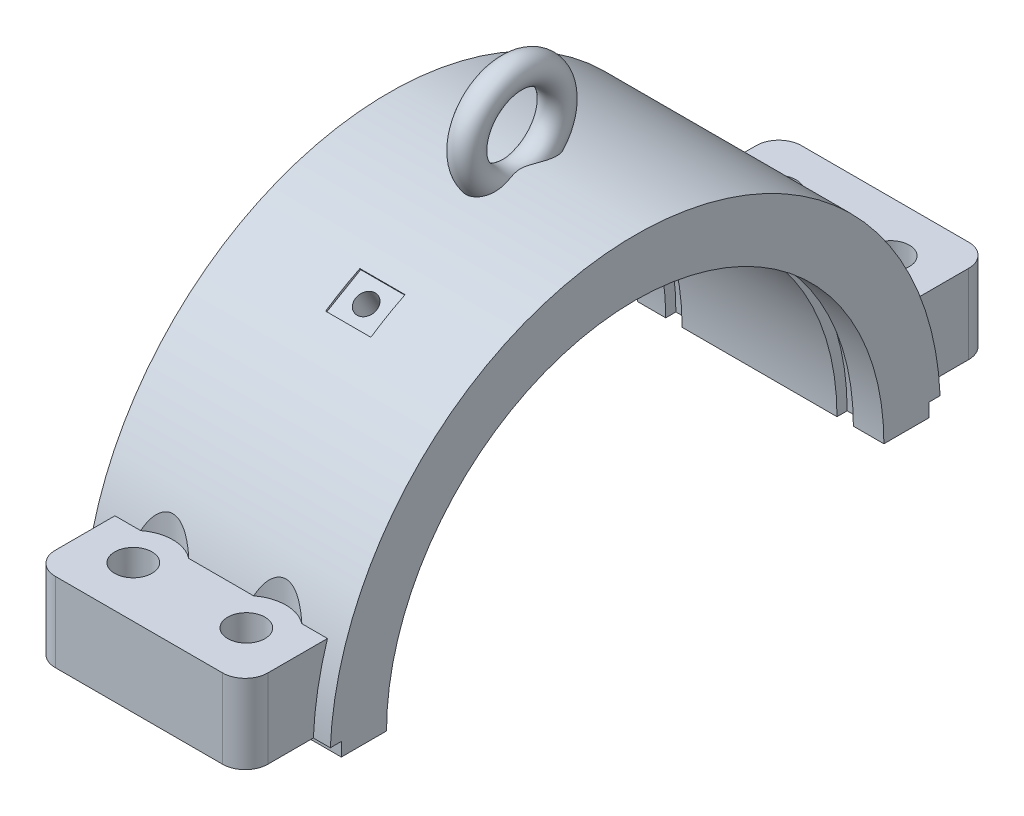
SolidWorks part; units mm, degrees
material "ZG270-500"
ref_plane "Front Plane" through (0, 0, 0) normal (0, 0, 1) x (1, 0, 0)
ref_plane "Top Plane" through (0, 0, 0) normal (0, 1, 0) x (1, 0, 0)
ref_plane "Right Plane" through (0, 0, 0) normal (1, 0, 0) x (0, 0, -1)
sketch "Sketch1" plane through (0, 0, 0) normal (1, 0, 0) x (0, 0, -1)
  line L0 (-323.4956, 0) -> (323.4956, 0) construction
  line L1 (0, 0) -> (0, 289.8169) construction
  line L2 (-270, 0) -> (-220, 0)
  line L3 (220, 0) -> (270, 0)
  arc A0 (220, 0) -> (-220, 0) centre (0, 0) ccw
  arc A1 (270, 0) -> (-270, 0) centre (0, 0) ccw
  point P3 (0, 0)
  dimension "D1" = 440
  dimension "D2" = 540
extrude "Boss-Extrude2" add sketch "Sketch1" along normal mid plane 218
sketch "Sketch4" plane through (0, 0, 0) normal (1, 0, 0) x (0, 0, -1)
  line L0 (-330, 12) -> (-269.7332, 12)
  line L1 (-330, 12) -> (-330, 82)
  line L2 (-330, 82) -> (-257.247, 82)
  line L3 (-270, 0) -> (-220, 0) construction
  line L4 (0, 0) -> (0, 117.0475) construction
  arc A0 (270, 0) -> (-270, 0) centre (0, 0) ccw construction
  arc A1 (-257.247, 82) -> (-269.7332, 12) centre (0, 0) ccw
  dimension "D1" = 12
  dimension "D2" = 70
  dimension "D3" = 330
extrude "Boss-Extrude3" add sketch "Sketch4" along normal mid plane 188
sketch "Sketch5" plane through (0, 82, 0) normal (0, 1, 0) x (1, 0, 0)
  line L0 (0, 0) -> (0, -285) construction
  line L1 (-50, -285) -> (50, -285) construction
  circle A0 centre (50, -285) radius 16.5
  circle A1 centre (-50, -285) radius 16.5
  point P5 (0, -285)
  dimension "D3" = 33
  dimension "D1" = 100
  dimension "D2" = 285
extrude "Cut-Extrude1" cut sketch "Sketch5" against normal through all both and the other way through all
sketch "Sketch6" plane through (0, 0, 0) normal (0, 1, 0) x (1, 0, 0)
  circle A0 centre (-50, -285) radius 35
  circle A1 centre (50, -285) radius 35
  dimension "D1" = 70
extrude "Cut-Extrude2" cut sketch "Sketch6" against normal up to surface (68 mm away) from offset 150
sketch "Sketch7" plane through (0, 0, 0) normal (1, 0, 0) x (0, 0, -1)
  line L0 (-299.2788, 12) -> (-260, 12)
  line L1 (-330, 12) -> (-269.7332, 12) construction
  line L2 (-260, 12) -> (-260, -5.7355)
  line L3 (-260, -5.7355) -> (-299.2788, -5.7355)
  line L4 (-299.2788, -5.7355) -> (-299.2788, 12)
  line L5 (0, 0) -> (0, -107.2673) construction
  dimension "D1" = 260
extrude "Cut-Extrude3" cut sketch "Sketch7" against normal through all both and the other way through all
fillet "Fillet1" radius 20 2 edges at (-94, 47, 330) (94, 47, 330)
mirror "Mirror1" about plane through (0, 0, 0) normal (0, 0, 1) of "Cut-Extrude3", "Boss-Extrude3", "Cut-Extrude1", "Cut-Extrude2", "Fillet1"
sketch "Sketch8" plane through (0, 0, 0) normal (0, 0, 1) x (1, 0, 0)
  line L0 (0, 0) -> (0, 229) construction
  line L1 (-84, 229) -> (-69.5, 229)
  line L2 (-69.5, 229) -> (-69.5, 220)
  line L3 (-69.5, 220) -> (-84, 220)
  line L4 (-84, 220) -> (-84, 229)
  line L6 (109, 0) -> (-109, 0) construction
  line L7 (82, 220) -> (82, 229)
  line L8 (67.5, 220) -> (82, 220)
  line L9 (67.5, 229) -> (67.5, 220)
  line L10 (82, 229) -> (67.5, 229)
  line L11 (0, 0) -> (171.999, 0) construction
  line L12 (109, 12) -> (109, 270) construction
  dimension "D1" = 27
  dimension "D2" = 14.5
  dimension "D3" = 220
  dimension "D4" = 229
  dimension "D5" = 166
  dimension "D6" = 14.5
revolve "Cut-Revolve1" cut sketch "Sketch8" angle 360 about L11
sketch "Sketch9" plane through (0, 0, 0) normal (0, 0, 1) x (1, 0, 0)
  line L0 (0, 0) -> (0, 300) construction
  line L1 (0, 300) -> (128.97, 300) construction
  line L2 (109, 0) -> (-109, 0) construction
  circle A0 centre (0, 340) radius 12.5
  dimension "D2" = 25
  dimension "D3" = 40
  dimension "D1" = 300
revolve "Revolve1" add sketch "Sketch9" angle 360 about L1
sketch "Sketch10" plane through (0, 0, 0) normal (1, 0, 0) x (0, 0, -1)
  line L0 (0, 0) -> (-135, 233.8269) construction
  line L1 (0, 0) -> (0, 321.2312) construction
  line L2 (-149.1554, 223.3448) -> (-118.8446, 240.8448)
  line L3 (-149.1554, 223.3448) -> (-151.1554, 226.8089)
  line L4 (-118.8446, 240.8448) -> (-120.8446, 244.3089)
  line L5 (-151.1554, 226.8089) -> (-120.8446, 244.3089)
  line L6 (-149.1554, 223.3448) -> (-120.8446, 244.3089) construction
  line L7 (-118.8446, 240.8448) -> (-151.1554, 226.8089) construction
  arc A0 (269.7332, 12) -> (-269.7332, 12) centre (0, 0) ccw construction
  dimension "D1" = 30
  dimension "D2" = 2
  dimension "D3" = 35
extrude "Cut-Extrude4" cut sketch "Sketch10" against normal mid plane 40 from offset 5
sketch "Sketch11" plane through (0, 232.0948, 134) normal (0, 0.866, 0.5) x (1, 0, 0)
  line L0 (5, 17.5) -> (5, 0) construction
  line L1 (-15, 17.5) -> (25, 17.5) construction
  line L2 (5, 0) -> (25, 0) construction
  line L3 (25, 17.5) -> (25, -17.5) construction
hole_wizard "M20x1.5 Tapped Hole1" positions "3DSketch1" profile "Sketch12" tap size "M20x1.5" standard "GB" end condition through all
sketch3d "3DSketch1"
  point P0 (5, 232.0948, 134)
cosmetic thread "hole cosmetic thread 1" parameters "D2"=20
sketch "Sketch12" plane through (5, 232.0948, 134) normal (1, 0, 0) x (0, -0.5, 0.866)
  line L0 (0, 0) -> (0, 433)
  line L1 (0, 433) -> (9.25, 433)
  line L2 (9.25, 433) -> (9.25, 0)
  line L5 (9.25, 0) -> (0, 0)
  line L11 (0, -6.35) -> (0, 107.95) construction
  dimension "通孔螺纹孔钻头直径" = 18.5
  dimension "通孔螺纹孔钻头深度" = 433
